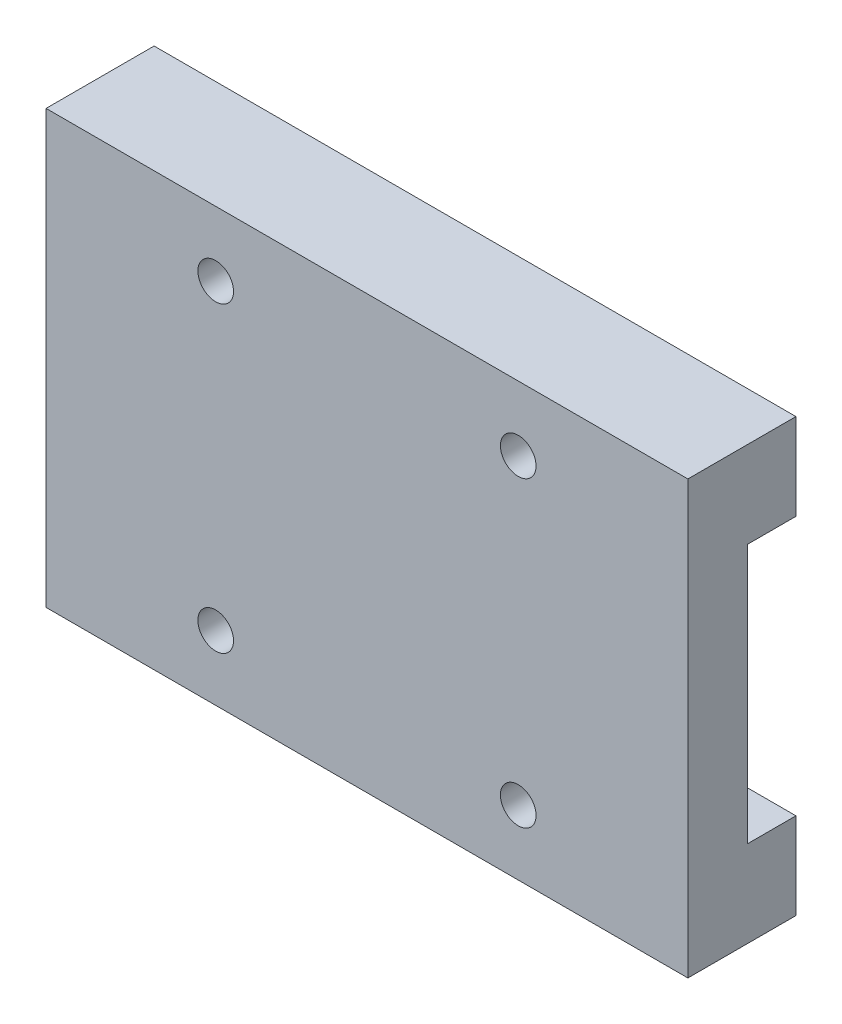
SolidWorks part; units mm, degrees
material "6061"
ref_plane "Front Plane" through (0, 0, 0) normal (0, 0, 1) x (1, 0, 0)
ref_plane "Top Plane" through (0, 0, 0) normal (0, 1, 0) x (1, 0, 0)
ref_plane "Right Plane" through (0, 0, 0) normal (1, 0, 0) x (0, 0, -1)
sketch "Sketch1" plane through (0, 0, 0) normal (0, 0, 1) x (1, 0, 0)
  line L1 (-29.7, 20) -> (29.7, 20)
  line L2 (-29.7, 20) -> (-29.7, -20)
  line L3 (-29.7, -20) -> (29.7, -20)
  line L4 (29.7, 20) -> (29.7, -20)
  line L5 (-29.7, 20) -> (29.7, -20) construction
  line L6 (-29.7, -20) -> (29.7, 20) construction
  point P0 (0, 0)
  dimension "D1" = 59.4
  dimension "D2" = 40
extrude "Boss-Extrude1" add sketch "Sketch1" along normal blind 10
sketch "Sketch2" plane through (-29.7, 0, 0) normal (-1, 0, 0) x (0, 0, 1)
  line L0 (0, 20) -> (0, -20) construction
  line L1 (-4.5, 12) -> (4.5, 12)
  line L2 (-4.5, 12) -> (-4.5, -12)
  line L3 (-4.5, -12) -> (4.5, -12)
  line L4 (4.5, 12) -> (4.5, -12)
  line L5 (-4.5, 12) -> (4.5, -12) construction
  line L6 (-4.5, -12) -> (4.5, 12) construction
  point P0 (0, 0)
  dimension "D1" = 24
  dimension "D2" = 4.5
extrude "Cut-Extrude1" cut sketch "Sketch2" against normal through all
hole_wizard "M4 Tapped Hole1" positions "Sketch4" profile "Sketch3" tap size "M4" standard "Gb"
sketch "Sketch4" plane through (0, 0, 10) normal (0, 0, 1) x (1, 0, 0)
  line L0 (-29.7, 0) -> (0, 0) construction
  line L1 (-29.7, 20) -> (-29.7, -20) construction
  line L2 (0, 0) -> (0, 20) construction
  line L3 (29.7, 20) -> (-29.7, 20) construction
  point P0 (-14, 14)
  point P16 (14, 14)
  point P17 (14, -14)
  point P18 (-14, -14)
  dimension "D1" = 14
  dimension "D2" = 14
sketch "Sketch3" plane through (-14, 14, 10) normal (1, 0, 0) x (0, -1, 0)
  line L0 (0, 0) -> (0, 11.0914)
  line L1 (0, 11.0914) -> (1.65, 10.1)
  line L2 (1.65, 10.1) -> (1.65, 0)
  line L5 (1.65, 0) -> (0, 0)
  line L10 (0, 11.0914) -> (-1.65, 10.1) construction
  line L11 (0, -6.35) -> (0, 107.95) construction
  dimension "螺纹孔钻头直径" = 3.3
  dimension "螺纹孔钻头深度" = 10.1
  dimension "导头角度" = 118
cosmetic thread "Hole thread1" parameters "D1"=8, "D2"=4
cosmetic thread "Hole thread2" parameters "D1"=8, "D2"=4
cosmetic thread "Hole thread3" parameters "D1"=8, "D2"=4
cosmetic thread "Hole thread4" parameters "D1"=8, "D2"=4
